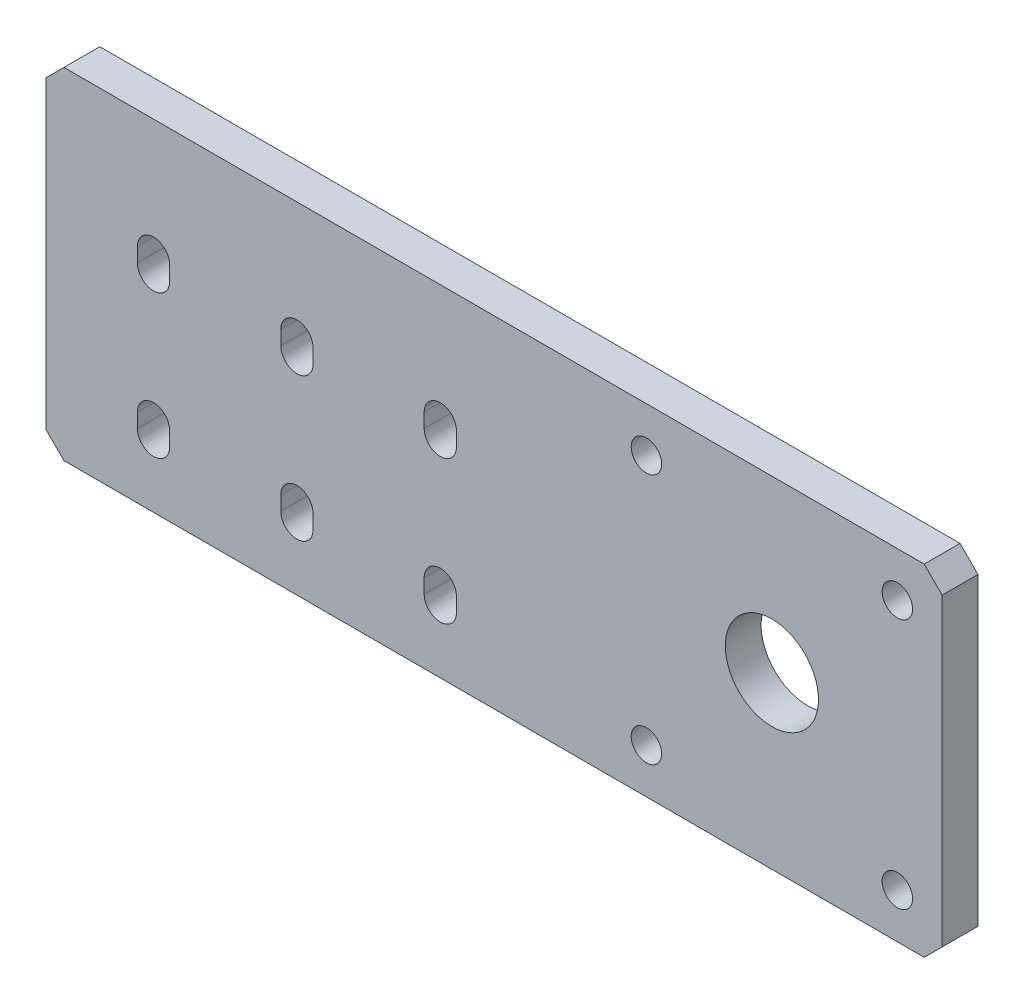
from build123d import *

# Parameters (mm, degrees)
SKETCH_1_W                  = 250
SKETCH_1_H                  = 95
EXTRUDE_1_DEPTH             = 10
CUT_EXTRUDE_2_DEPTH         = 135.094183319
PATTERN_LINEAR_1_COUNT      = 2
PATTERN_LINEAR_1_PITCH      = 40
PATTERN_LINEAR_1_COUNT_DIR2 = 2
PATTERN_LINEAR_1_PITCH_DIR2 = 40
PATTERN_LINEAR_2_COUNT      = 2
PATTERN_LINEAR_2_PITCH      = 40
PATTERN_LINEAR_2_COUNT_DIR2 = 2
PATTERN_LINEAR_2_PITCH_DIR2 = 40
CHAMFER_1_SIZE              = 5
HOLE_WIZARD_M10_3_D         = 8.5
HOLE_WIZARD_M10_3_DEPTH     = 24.5
HOLE_WIZARD_M10_3_TIP       = 2.553657631
SKETCH_12_R                 = 13
CUT_EXTRUDE_5_DEPTH         = 135.094183319
HOLE_WIZARD_M4_1_D          = 3.3
HOLE_WIZARD_M4_1_DEPTH      = 10.1
HOLE_WIZARD_M4_1_TIP        = 0.991420021


with BuildPart() as part:
    # 草图1 → 凸台-拉伸1 (new body)
    with BuildSketch(Plane.XY):
        Rectangle(SKETCH_1_W, SKETCH_1_H)
    extrude(amount=EXTRUDE_1_DEPTH)

    # 草图3 → 切除-拉伸2 (cut, through all)
    with BuildSketch(Plane.XY.offset(10)):
        with BuildLine():
            Line((-59.5, -29.5), (-59.5, -25.5))
            ThreePointArc((-59.5, -25.5), (-55, -21), (-50.5, -25.5))
            Line((-50.5, -25.5), (-50.5, -29.5))
            ThreePointArc((-50.5, -29.5), (-55, -34), (-59.5, -29.5))
        make_face()
    cut_extrude_2 = extrude(amount=-CUT_EXTRUDE_2_DEPTH, mode=Mode.SUBTRACT)

    # 阵列(线性)1: Cut-Extrude 2 2 × 2
    with Locations(*[(i * PATTERN_LINEAR_1_PITCH, j * PATTERN_LINEAR_1_PITCH_DIR2, 0) for i in range(PATTERN_LINEAR_1_COUNT) for j in range(PATTERN_LINEAR_1_COUNT_DIR2) if (i, j) != (0, 0)]):
        add(cut_extrude_2, mode=Mode.SUBTRACT)

    # 阵列(线性)2: Cut-Extrude 2 2 × 2
    with Locations(*[(-i * PATTERN_LINEAR_2_PITCH, j * PATTERN_LINEAR_2_PITCH_DIR2, 0) for i in range(PATTERN_LINEAR_2_COUNT) for j in range(PATTERN_LINEAR_2_COUNT_DIR2) if (i, j) != (0, 0)]):
        add(cut_extrude_2, mode=Mode.SUBTRACT)

    # 倒角1
    chamfer_1_edges = [part.edges().sort_by_distance(p)[0] for p in [
        (125, -47.5, 5),
        (-125, -47.5, 5),
        (-125, 47.5, 5),
        (125, 47.5, 5),
    ]]
    chamfer(chamfer_1_edges, length=CHAMFER_1_SIZE)

    # M10 螺纹孔3
    with Locations(Plane(origin=(42.5, 35, 10), x_dir=(1, 0, 0), z_dir=(0, 0, 1))):
        with Locations((0, 0), (70, 0), (70, -70), (0, -70)):
            Hole(HOLE_WIZARD_M10_3_D / 2, depth=HOLE_WIZARD_M10_3_DEPTH)
            with Locations((0, 0, -(HOLE_WIZARD_M10_3_DEPTH + HOLE_WIZARD_M10_3_TIP / 2))):  # 118° drill point
                Cone(0, HOLE_WIZARD_M10_3_D / 2, HOLE_WIZARD_M10_3_TIP, mode=Mode.SUBTRACT)

    # 草图12 → 切除-拉伸5 (cut, through all)
    with BuildSketch(Plane.XY.offset(10)):
        with Locations((77.5, 0)):
            Circle(SKETCH_12_R)
    extrude(amount=-CUT_EXTRUDE_5_DEPTH, mode=Mode.SUBTRACT)

    # M4 螺纹孔1
    with Locations(Plane(origin=(117, -47.5, 5), x_dir=(0, 0, -1), z_dir=(0, -1, 0))):
        with Locations((0, 0), (0, -105), (0, -52.5)):
            Hole(HOLE_WIZARD_M4_1_D / 2, depth=HOLE_WIZARD_M4_1_DEPTH)
            with Locations((0, 0, -(HOLE_WIZARD_M4_1_DEPTH + HOLE_WIZARD_M4_1_TIP / 2))):  # 118° drill point
                Cone(0, HOLE_WIZARD_M4_1_D / 2, HOLE_WIZARD_M4_1_TIP, mode=Mode.SUBTRACT)


solid = part.part
